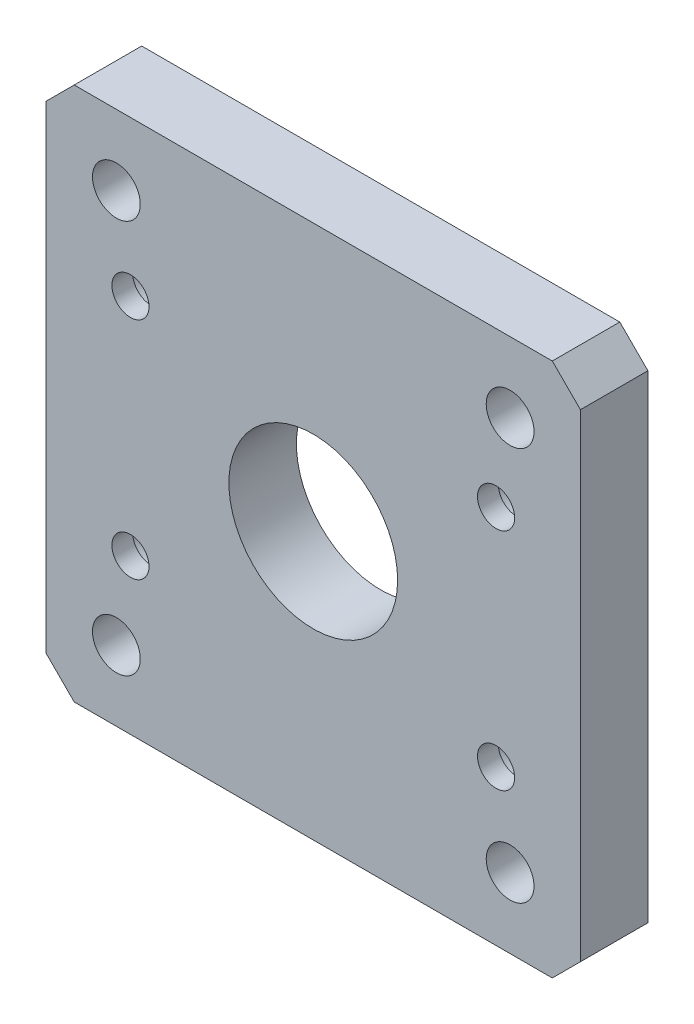
SolidWorks part; units mm, degrees
material "AISI 1045 钢，冷拔"
ref_plane "前视基准面" through (0, 0, 0) normal (0, 0, 1) x (1, 0, 0)
ref_plane "上视基准面" through (0, 0, 0) normal (0, 1, 0) x (1, 0, 0)
ref_plane "右视基准面" through (0, 0, 0) normal (1, 0, 0) x (0, 0, -1)
sketch "草图1" plane through (0, 0, 0) normal (0, 0, 1) x (1, 0, 0)
  line L0 (-70, -47.5) -> (90, -47.5) construction
  line L1 (0.8045, -47.5) -> (95.8045, -47.5)
  line L2 (0.8045, -47.5) -> (0.8045, 47.5)
  line L3 (0.8045, 47.5) -> (95.8045, 47.5)
  line L4 (95.8045, -47.5) -> (95.8045, 47.5)
  dimension "D1" = 95
  dimension "D2" = 95
extrude "凸台-拉伸1" add sketch "草图1" along normal blind 12
sketch "草图2" plane through (0, 0, 12) normal (0, 0, 1) x (1, 0, 0)
  line L0 (48.3045, 47.5) -> (48.3045, -47.5) construction
  line L1 (95.8045, 47.5) -> (0.8045, 47.5) construction
  line L2 (0.8045, -47.5) -> (95.8045, -47.5) construction
  circle A0 centre (48.3045, 0) radius 15
  dimension "D1" = 30
extrude "切除-拉伸1" cut sketch "草图2" against normal through all
sketch "草图3" [suppressed] plane through (0, 0, 10) normal (0, 0, 1) x (1, 0, 0)
  point P0 (16.3045, 32)
  point P1 (80.3045, 32)
  point P3 (80.3045, -32)
  point P5 (16.3045, -32)
hole_wizard "M10 螺纹孔1" positions "3D草图1" profile "草图4" tap size "M10" standard "GB"
sketch3d "3D草图1" [suppressed]
  point P0 (80.3045, 32, 10)
  point P3 (80.3045, -32, 10)
  point P6 (16.3045, -32, 10)
  point P9 (16.3045, 32, 10)
sketch "草图4" plane through (80.3045, 32, 10) normal (1, 0, 0) x (0, -1, 0)
  line L0 (0, 0) -> (0, 27.0537)
  line L1 (0, 27.0537) -> (4.25, 24.5)
  line L2 (4.25, 24.5) -> (4.25, 0)
  line L5 (4.25, 0) -> (0, 0)
  line L10 (0, 27.0537) -> (-4.25, 24.5) construction
  line L11 (0, -6.35) -> (0, 107.95) construction
  dimension "螺纹孔钻头直径" = 8.5
  dimension "螺纹孔钻头深度" = 24.5
  dimension "导头角度" = 118
cosmetic thread "孔螺蚊线1" [suppressed] parameters "D1"=10, "D2"=10
cosmetic thread "孔螺蚊线2" [suppressed] parameters "D1"=10, "D2"=10
cosmetic thread "孔螺蚊线3" [suppressed] parameters "D1"=10, "D2"=10
cosmetic thread "孔螺蚊线4" [suppressed] parameters "D1"=10, "D2"=10
sketch "草图5" plane through (0, 0, 0) normal (0, 0, -1) x (-1, 0, 0)
  line L5 (-15.8045, 20) -> (-80.8045, 20) construction
  line L6 (-15.8045, 20) -> (-15.8045, -20) construction
  line L7 (-15.8045, -20) -> (-80.8045, -20) construction
  line L8 (-80.8045, 20) -> (-80.8045, -20) construction
  line L9 (-15.8045, 20) -> (-80.8045, -20) construction
  line L10 (-15.8045, -20) -> (-80.8045, 20) construction
  point P7 (-48.3045, 0)
  dimension "D1" = 65
  dimension "D2" = 40
hole_wizard "打孔尺寸(%根据)内六角圆柱头螺钉的类型1" positions "3D草图11" profile "草图10" counterbore size "M6" standard "GB" end condition through all
sketch3d "3D草图11"
  point P0 (80.8045, 20, 0)
  point P3 (15.8045, 20, 0)
  point P6 (15.8045, -20, 0)
  point P9 (80.8045, -20, 0)
sketch "草图10" plane through (80.8045, 20, 0) normal (1, 0, 0) x (0, 1, 0)
  line L0 (0, 0) -> (0, 12)
  line L1 (0, 12) -> (3.3, 12)
  line L3 (3.3, 12) -> (3.3, 8.3)
  line L4 (3.3, 8.3) -> (5.5, 8.3)
  line L5 (5.5, 8.3) -> (5.5, 0)
  line L7 (5.5, 0) -> (0, 0)
  line L11 (0, -6.35) -> (0, 107.95) construction
  dimension "通孔孔直径" = 6.6
  dimension "通孔孔深度" = 12
  dimension "柱形沉头孔直径" = 11
  dimension "柱形沉头孔深度" = 8.3
sketch "草图11" plane through (0, 0, 0) normal (0, 0, -1) x (-1, 0, 0)
  line L0 (-15.8045, 20) -> (-80.8045, -20) construction
  line L1 (-83.3045, 35) -> (-13.3045, 35) construction
  line L2 (-83.3045, 35) -> (-83.3045, -35) construction
  line L3 (-83.3045, -35) -> (-13.3045, -35) construction
  line L4 (-13.3045, 35) -> (-13.3045, -35) construction
  line L5 (-83.3045, 35) -> (-13.3045, -35) construction
  line L6 (-83.3045, -35) -> (-13.3045, 35) construction
  point P0 (-48.3045, 0)
  dimension "D1" = 70
  dimension "D2" = 70
hole_wizard "M10 螺纹孔2" positions "3D草图12" profile "草图12" tap size "M10" standard "GB" end condition through all
sketch3d "3D草图12"
  point P0 (83.3045, 35, 0)
  point P3 (13.3045, 35, 0)
  point P6 (13.3045, -35, 0)
  point P9 (83.3045, -35, 0)
cosmetic thread "孔螺蚊线21" parameters "D2"=10
cosmetic thread "孔螺蚊线22" parameters "D2"=10
cosmetic thread "孔螺蚊线23" parameters "D2"=10
cosmetic thread "孔螺蚊线24" parameters "D2"=10
sketch "草图12" plane through (83.3045, 35, 0) normal (1, 0, 0) x (0, 1, 0)
  line L0 (0, 0) -> (0, 12)
  line L1 (0, 12) -> (4.25, 12)
  line L2 (4.25, 12) -> (4.25, 0)
  line L5 (4.25, 0) -> (0, 0)
  line L11 (0, -6.35) -> (0, 107.95) construction
  dimension "通孔螺纹孔钻头直径" = 8.5
  dimension "通孔螺纹孔钻头深度" = 12
chamfer "倒角1" distance 5 angle 45 4 edges at (95.8045, 47.5, 6) (95.8045, -47.5, 6) (0.8045, 47.5, 6) (0.8045, -47.5, 6)
